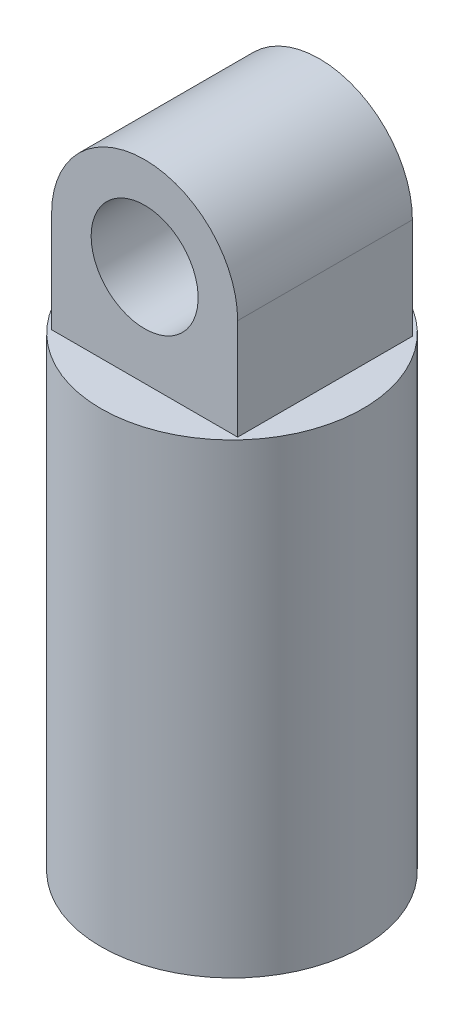
SolidWorks part; units mm, degrees
ref_plane "Front Plane" through (0, 0, 0) normal (0, 0, 1) x (1, 0, 0)
ref_plane "Top Plane" through (0, 0, 0) normal (0, 1, 0) x (1, 0, 0)
ref_plane "Right Plane" through (0, 0, 0) normal (1, 0, 0) x (0, 0, -1)
other "Configuration Table"
sketch "Sketch2" plane through (0, 0, 10.6078) normal (0, 0, -1) x (-1, 0, 0)
  line L0 (20.8001, -16.2883) -> (20.8001, -23.2153)
  line L1 (20.8001, -23.2153) -> (33.5776, -23.2153)
  line L2 (33.5776, -23.2153) -> (33.5776, -16.2883)
  arc A0 (33.5776, -16.2883) -> (20.8001, -16.2883) centre (27.1889, -16.2883) ccw
extrude "Boss-Extrude1" add sketch "Sketch2" along normal mid plane 12
sketch "Sketch3" plane through (0, -23.2153, 0) normal (0, -1, 0) x (1, 0, 0)
  circle A0 centre (-27.1889, 10.6078) radius 9
extrude "Boss-Extrude2" add sketch "Sketch3" along normal blind 32
sketch "Sketch5" plane through (0, 0, 4.6078) normal (0, 0, -1) x (-1, 0, 0)
  circle A1 centre (27.1889, -16.2883) radius 3.6746
extrude "Cut-Extrude1" cut sketch "Sketch5" against normal up to surface (12 mm away) up to face at (-27.1889, -18.1546, 16.6078)
